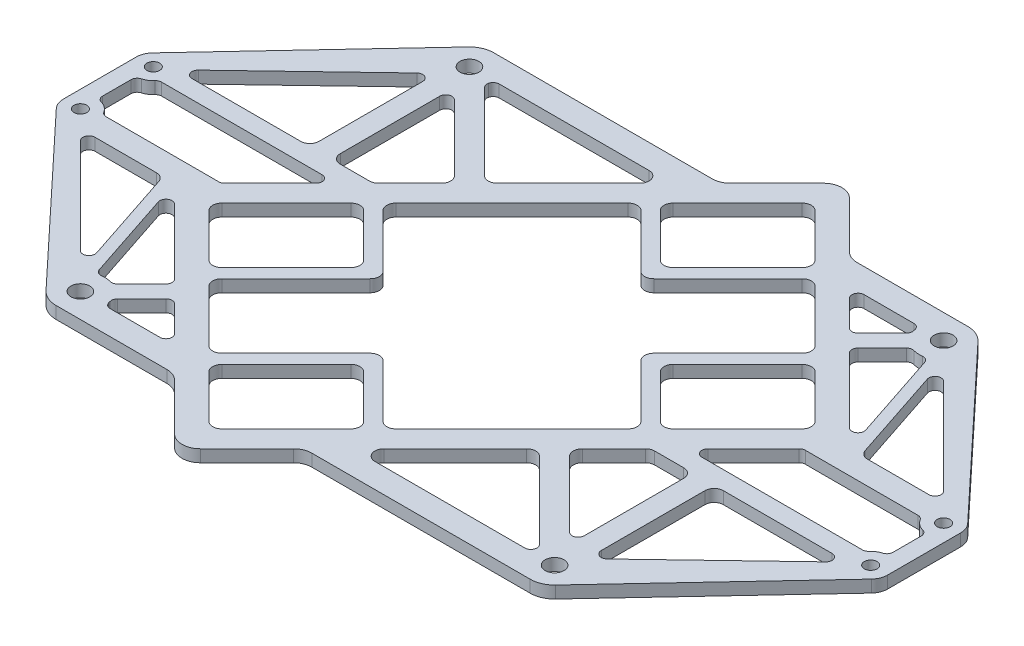
from build123d import *

# Parameters (mm, degrees)
SKETCH_1_R      = 2.8
SKETCH_1_R_2    = 1.05
SKETCH_1_R_3    = 4
SKETCH_1_R_4    = 1.55
EXTRUDE_1_DEPTH = 2
EXTRUDE_2_DEPTH = 2
FILLET_1_5_R    = 1.5
FILLET_1_R      = 1
FILLET_3_R      = 3


with BuildPart() as part:
    # 草图1 → 凸台-拉伸1 (new body)
    # profile 1 of 33: a face of its own
    with BuildSketch(Plane(origin=(0, 0, 0), x_dir=(1, 0, 0), z_dir=(0, 1, 0))):
        with BuildLine():
            ThreePointArc((-65, 3.2), (-66.979898987, 4.020101013), (-67.8, 6))
            Line((-67.8, 6), (-67.8, -6))
            ThreePointArc((-67.8, -6), (-66.979898987, -4.020101013), (-65, -3.2))
            Line((-65, -3.2), (-65, 3.2))
        make_face()
    # profile 2 of 33: a face of its own
    with BuildSketch(Plane(origin=(0, 0, 0), x_dir=(1, 0, 0), z_dir=(0, 1, 0))):
        with Locations((-65, 6)):
            Circle(SKETCH_1_R)
        with Locations(Location((-65, 6, 0), (0, 0, 270))):
            Circle(SKETCH_1_R_2, mode=Mode.SUBTRACT)
    # profile 3 of 33: a face of its own
    with BuildSketch(Plane(origin=(0, 0, 0), x_dir=(1, 0, 0), z_dir=(0, 1, 0))):
        with BuildLine():
            ThreePointArc((-40.75, 28.403126358), (-42.933491188, 31.273606806), (-41.919228153, 34.734612768))
            Line((-41.919228153, 34.734612768), (-67.043459707, 7.914228938))
            ThreePointArc((-67.043459707, 7.914228938), (-64.738019223, 8.787717), (-62.635681916, 7.5))
            Line((-62.635681916, 7.5), (-40.75, 28.403126358))
        make_face()
    # profile 4 of 33: a face of its own
    with BuildSketch(Plane(origin=(0, 0, 0), x_dir=(1, 0, 0), z_dir=(0, 1, 0))):
        with BuildLine():
            Line((-33.330212793, 4.5), (-30.330212793, 7.5))
            Line((-30.330212793, 7.5), (-37.25, 7.5))
            Line((-37.25, 7.5), (-40.75, 7.5))
            Line((-40.75, 7.5), (-62.635681916, 7.5))
            ThreePointArc((-62.635681916, 7.5), (-62.311125641, 6.780995956), (-62.2, 6))
            ThreePointArc((-62.2, 6), (-62.311125641, 5.219004044), (-62.635681916, 4.5))
            Line((-62.635681916, 4.5), (-33.330212793, 4.5))
        make_face()
    # profile 5 of 33: a face of its own
    with BuildSketch(Plane(origin=(0, 0, 0), x_dir=(1, 0, 0), z_dir=(0, 1, 0))):
        with Locations((-65, -6)):
            Circle(SKETCH_1_R)
        with Locations(Location((-65, -6, 0), (0, 0, 270))):
            Circle(SKETCH_1_R_2, mode=Mode.SUBTRACT)
    # profile 6 of 33: a face of its own
    with BuildSketch(Plane(origin=(0, 0, 0), x_dir=(1, 0, 0), z_dir=(0, 1, 0))):
        with BuildLine():
            Line((-46.669047558, -8.838834765), (-42.830212793, -5))
            Line((-42.830212793, -5), (-62.384660634, -5))
            ThreePointArc((-62.384660634, -5), (-62.246552141, -5.491546573), (-62.2, -6))
            ThreePointArc((-62.2, -6), (-62.413137309, -7.071513611), (-63.020101013, -7.979898987))
            Line((-63.020101013, -7.979898987), (-62.161165235, -8.838834765))
            Line((-62.161165235, -8.838834765), (-48.560935355, -8.838834765))
            Line((-48.560935355, -8.838834765), (-46.669047558, -8.838834765))
        make_face()
    # profile 7 of 33: a face of its own
    with BuildSketch(Plane(origin=(0, 0, 0), x_dir=(1, 0, 0), z_dir=(0, 1, 0))):
        with BuildLine():
            Line((-67.043459707, -7.914228938), (-41.919228153, -34.734612768))
            ThreePointArc((-41.919228153, -34.734612768), (-42.999467278, -31.934719911), (-41.828427125, -29.171572875))
            Line((-41.828427125, -29.171572875), (-62.161165235, -8.838834765))
            Line((-62.161165235, -8.838834765), (-63.020101013, -7.979898987))
            ThreePointArc((-63.020101013, -7.979898987), (-65.045696062, -8.799627095), (-67.043459707, -7.914228938))
        make_face()
    # profile 8 of 33: a face of its own
    with BuildSketch(Plane(origin=(0, 0, 0), x_dir=(1, 0, 0), z_dir=(0, 1, 0))):
        with BuildLine():
            Line((-48.560935355, -8.838834765), (-41.828427125, -29.171572875))
            ThreePointArc((-41.828427125, -29.171572875), (-41.099527033, -28.595299391), (-40.257332988, -28.202749184))
            Line((-40.257332988, -28.202749184), (-46.669047558, -8.838834765))
            Line((-46.669047558, -8.838834765), (-48.560935355, -8.838834765))
        make_face()
    # profile 9 of 33: a face of its own
    with BuildSketch(Plane(origin=(0, 0, 0), x_dir=(1, 0, 0), z_dir=(0, 1, 0))):
        Polygon((46.669047558, 8.838834765), (8.838834765, 46.669047558), (-46.669047558, -8.838834765), (-8.838834765, -46.669047558), align=None)
        Polygon((41.012193309, 8.838834765), (8.838834765, 41.012193309), (-41.012193309, -8.838834765), (-8.838834765, -41.012193309), align=None, mode=Mode.SUBTRACT)
    # profile 10 of 33: a face of its own
    with BuildSketch(Plane(origin=(0, 0, 0), x_dir=(1, 0, 0), z_dir=(0, 1, 0))):
        with Locations((-39, 32)):
            Circle(SKETCH_1_R_3)
        with Locations(Location((-39, 32, 0), (0, 0, 270))):
            Circle(SKETCH_1_R_4, mode=Mode.SUBTRACT)
    # profile 11 of 33: a face of its own
    with BuildSketch(Plane(origin=(0, 0, 0), x_dir=(1, 0, 0), z_dir=(0, 1, 0))):
        with BuildLine():
            ThreePointArc((-37.694063123, 28.219189389), (-39.240325231, 28.007226054), (-40.75, 28.403126358))
            Line((-40.75, 28.403126358), (-40.75, 7.5))
            Line((-40.75, 7.5), (-37.25, 7.5))
            Line((-37.25, 7.5), (-37.25, 27.775126266))
            Line((-37.25, 27.775126266), (-37.694063123, 28.219189389))
        make_face()
    # profile 12 of 33: a face of its own
    with BuildSketch(Plane(origin=(0, 0, 0), x_dir=(1, 0, 0), z_dir=(0, 1, 0))):
        with BuildLine():
            Line((-37.694063123, 28.219189389), (-37.25, 27.775126266))
            Line((-37.25, 27.775126266), (-37.25, 28.403126358))
            ThreePointArc((-37.25, 28.403126358), (-37.469266271, 28.30448187), (-37.694063123, 28.219189389))
        make_face()
    # profile 13 of 33: a face of its own
    with BuildSketch(Plane(origin=(0, 0, 0), x_dir=(1, 0, 0), z_dir=(0, 1, 0))):
        with BuildLine():
            Line((-23.652543264, 14.17766953), (-21.17766953, 16.652543264))
            Line((-21.17766953, 16.652543264), (-35.219189389, 30.694063123))
            ThreePointArc((-35.219189389, 30.694063123), (-36.006746867, 29.346618067), (-37.25, 28.403126358))
            Line((-37.25, 28.403126358), (-37.25, 27.775126266))
            Line((-37.25, 27.775126266), (-23.652543264, 14.17766953))
        make_face()
    # profile 14 of 33: a face of its own
    with BuildSketch(Plane(origin=(0, 0, 0), x_dir=(1, 0, 0), z_dir=(0, 1, 0))):
        with BuildLine():
            Line((-5.830212793, 32), (-1.830212793, 36))
            Line((-1.830212793, 36), (-39, 36))
            ThreePointArc((-39, 36), (-36.171572875, 34.828427125), (-35, 32))
            Line((-35, 32), (-5.830212793, 32))
        make_face()
    # profile 15 of 33: a face of its own
    with BuildSketch(Plane(origin=(0, 0, 0), x_dir=(1, 0, 0), z_dir=(0, 1, 0))):
        with Locations((-39, -32)):
            Circle(SKETCH_1_R_3)
        with Locations(Location((-39, -32, 0), (0, 0, 270))):
            Circle(SKETCH_1_R_4, mode=Mode.SUBTRACT)
    # profile 16 of 33: a face of its own
    with BuildSketch(Plane(origin=(0, 0, 0), x_dir=(1, 0, 0), z_dir=(0, 1, 0))):
        with BuildLine():
            Line((-35.317317708, -30.438638051), (-30.19328099, -25.314601333))
            Line((-30.19328099, -25.314601333), (-32.314601333, -23.19328099))
            Line((-32.314601333, -23.19328099), (-37.438638051, -28.317317708))
            ThreePointArc((-37.438638051, -28.317317708), (-36.171572875, -29.171572875), (-35.317317708, -30.438638051))
        make_face()
    # profile 17 of 33: a face of its own
    with BuildSketch(Plane(origin=(0, 0, 0), x_dir=(1, 0, 0), z_dir=(0, 1, 0))):
        with BuildLine():
            Line((-39, -36), (-19.507882323, -36))
            Line((-19.507882323, -36), (-23.507882323, -32))
            Line((-23.507882323, -32), (-35, -32))
            ThreePointArc((-35, -32), (-36.171572875, -34.828427125), (-39, -36))
        make_face()
    # profile 18 of 33: a face of its own
    with BuildSketch(Plane(origin=(0, 0, 0), x_dir=(1, 0, 0), z_dir=(0, 1, 0))):
        with BuildLine():
            Line((35, -32), (5.830212793, -32))
            Line((5.830212793, -32), (1.830212793, -36))
            Line((1.830212793, -36), (39, -36))
            ThreePointArc((39, -36), (36.171572875, -34.828427125), (35, -32))
        make_face()
    # profile 19 of 33: a face of its own
    with BuildSketch(Plane(origin=(0, 0, 0), x_dir=(1, 0, 0), z_dir=(0, 1, 0))):
        with BuildLine():
            Line((37.25, -27.775126266), (23.652543264, -14.17766953))
            Line((23.652543264, -14.17766953), (21.17766953, -16.652543264))
            Line((21.17766953, -16.652543264), (35.219189389, -30.694063123))
            ThreePointArc((35.219189389, -30.694063123), (36.006746867, -29.346618067), (37.25, -28.403126358))
            Line((37.25, -28.403126358), (37.25, -27.775126266))
        make_face()
    # profile 20 of 33: a face of its own
    with BuildSketch(Plane(origin=(0, 0, 0), x_dir=(1, 0, 0), z_dir=(0, 1, 0))):
        with BuildLine():
            Line((40.75, -7.5), (37.25, -7.5))
            Line((37.25, -7.5), (37.25, -27.775126266))
            Line((37.25, -27.775126266), (37.694063123, -28.219189389))
            ThreePointArc((37.694063123, -28.219189389), (39.240325231, -28.007226054), (40.75, -28.403126358))
            Line((40.75, -28.403126358), (40.75, -7.5))
        make_face()
    # profile 21 of 33: a face of its own
    with BuildSketch(Plane(origin=(0, 0, 0), x_dir=(1, 0, 0), z_dir=(0, 1, 0))):
        with Locations((39, -32)):
            Circle(SKETCH_1_R_3)
        with Locations(Location((39, -32, 0), (0, 0, 270))):
            Circle(SKETCH_1_R_4, mode=Mode.SUBTRACT)
    # profile 22 of 33: a face of its own
    with BuildSketch(Plane(origin=(0, 0, 0), x_dir=(1, 0, 0), z_dir=(0, 1, 0))):
        with BuildLine():
            Line((37.694063123, -28.219189389), (37.25, -27.775126266))
            Line((37.25, -27.775126266), (37.25, -28.403126358))
            ThreePointArc((37.25, -28.403126358), (37.469266271, -28.30448187), (37.694063123, -28.219189389))
        make_face()
    # profile 23 of 33: a face of its own
    with BuildSketch(Plane(origin=(0, 0, 0), x_dir=(1, 0, 0), z_dir=(0, 1, 0))):
        with BuildLine():
            ThreePointArc((67.043459707, -7.914228938), (64.738019223, -8.787717), (62.635681916, -7.5))
            Line((62.635681916, -7.5), (40.75, -28.403126358))
            ThreePointArc((40.75, -28.403126358), (42.391164992, -29.878679656), (43, -32))
            ThreePointArc((43, -32), (42.720007568, -33.470218927), (41.919228153, -34.734612768))
            Line((41.919228153, -34.734612768), (67.043459707, -7.914228938))
        make_face()
    # profile 24 of 33: a face of its own
    with BuildSketch(Plane(origin=(0, 0, 0), x_dir=(1, 0, 0), z_dir=(0, 1, 0))):
        with Locations((65, -6)):
            Circle(SKETCH_1_R)
        with Locations(Location((65, -6, 0), (0, 0, 270))):
            Circle(SKETCH_1_R_2, mode=Mode.SUBTRACT)
    # profile 25 of 33: a face of its own
    with BuildSketch(Plane(origin=(0, 0, 0), x_dir=(1, 0, 0), z_dir=(0, 1, 0))):
        with BuildLine():
            Line((62.635681916, -4.5), (33.330212793, -4.5))
            Line((33.330212793, -4.5), (30.330212793, -7.5))
            Line((30.330212793, -7.5), (37.25, -7.5))
            Line((37.25, -7.5), (40.75, -7.5))
            Line((40.75, -7.5), (62.635681916, -7.5))
            ThreePointArc((62.635681916, -7.5), (62.2, -6), (62.635681916, -4.5))
        make_face()
    # profile 26 of 33: a face of its own
    with BuildSketch(Plane(origin=(0, 0, 0), x_dir=(1, 0, 0), z_dir=(0, 1, 0))):
        with BuildLine():
            ThreePointArc((67.8, 6), (66.979898987, 4.020101013), (65, 3.2))
            Line((65, 3.2), (65, -3.2))
            ThreePointArc((65, -3.2), (66.979898987, -4.020101013), (67.8, -6))
            Line((67.8, -6), (67.8, 6))
        make_face()
    # profile 27 of 33: a face of its own
    with BuildSketch(Plane(origin=(0, 0, 0), x_dir=(1, 0, 0), z_dir=(0, 1, 0))):
        with BuildLine():
            Line((48.560935355, 8.838834765), (46.669047558, 8.838834765))
            Line((46.669047558, 8.838834765), (42.830212793, 5))
            Line((42.830212793, 5), (62.384660634, 5))
            ThreePointArc((62.384660634, 5), (62.261569177, 6.583949163), (63.020101013, 7.979898987))
            Line((63.020101013, 7.979898987), (62.161165235, 8.838834765))
            Line((62.161165235, 8.838834765), (48.560935355, 8.838834765))
        make_face()
    # profile 28 of 33: a face of its own
    with BuildSketch(Plane(origin=(0, 0, 0), x_dir=(1, 0, 0), z_dir=(0, 1, 0))):
        with BuildLine():
            Line((41.828427125, 29.171572875), (62.161165235, 8.838834765))
            Line((62.161165235, 8.838834765), (63.020101013, 7.979898987))
            ThreePointArc((63.020101013, 7.979898987), (65.045696062, 8.799627095), (67.043459707, 7.914228938))
            Line((67.043459707, 7.914228938), (41.919228153, 34.734612768))
            ThreePointArc((41.919228153, 34.734612768), (42.720007568, 33.470218927), (43, 32))
            ThreePointArc((43, 32), (42.69551813, 30.469266271), (41.828427125, 29.171572875))
        make_face()
    # profile 29 of 33: a face of its own
    with BuildSketch(Plane(origin=(0, 0, 0), x_dir=(1, 0, 0), z_dir=(0, 1, 0))):
        with Locations((65, 6)):
            Circle(SKETCH_1_R)
        with Locations(Location((65, 6, 0), (0, 0, 270))):
            Circle(SKETCH_1_R_2, mode=Mode.SUBTRACT)
    # profile 30 of 33: a face of its own
    with BuildSketch(Plane(origin=(0, 0, 0), x_dir=(1, 0, 0), z_dir=(0, 1, 0))):
        with BuildLine():
            Line((40.257332988, 28.202749184), (46.669047558, 8.838834765))
            Line((46.669047558, 8.838834765), (48.560935355, 8.838834765))
            Line((48.560935355, 8.838834765), (41.828427125, 29.171572875))
            ThreePointArc((41.828427125, 29.171572875), (41.099527033, 28.595299391), (40.257332988, 28.202749184))
        make_face()
    # profile 31 of 33: a face of its own
    with BuildSketch(Plane(origin=(0, 0, 0), x_dir=(1, 0, 0), z_dir=(0, 1, 0))):
        with BuildLine():
            Line((19.507882323, 36), (23.507882323, 32))
            Line((23.507882323, 32), (35, 32))
            ThreePointArc((35, 32), (36.171572875, 34.828427125), (39, 36))
            Line((39, 36), (19.507882323, 36))
        make_face()
    # profile 32 of 33: a face of its own
    with BuildSketch(Plane(origin=(0, 0, 0), x_dir=(1, 0, 0), z_dir=(0, 1, 0))):
        with Locations((39, 32)):
            Circle(SKETCH_1_R_3)
        with Locations(Location((39, 32, 0), (0, 0, 270))):
            Circle(SKETCH_1_R_4, mode=Mode.SUBTRACT)
    # profile 33 of 33: a face of its own
    with BuildSketch(Plane(origin=(0, 0, 0), x_dir=(1, 0, 0), z_dir=(0, 1, 0))):
        with BuildLine():
            Line((30.19328099, 25.314601333), (32.314601333, 23.19328099))
            Line((32.314601333, 23.19328099), (37.438638051, 28.317317708))
            ThreePointArc((37.438638051, 28.317317708), (36.171572875, 29.171572875), (35.317317708, 30.438638051))
            Line((35.317317708, 30.438638051), (30.19328099, 25.314601333))
        make_face()
    extrude(amount=EXTRUDE_1_DEPTH)

    # 草图2 → 凸台-拉伸2 (add)
    with BuildSketch(Plane(origin=(0, 2, 0), x_dir=(1, 0, 0), z_dir=(0, 1, 0))):
        Polygon((-3.889087297, 28.284271247), (5.303300859, 19.091883092), (18.03122292, 31.819805153), (19.622213178, 30.228814896), (5.303300859, 15.909902577), (-5.480077554, 26.69328099), align=None)
        Polygon((-31.819805153, -18.03122292), (-30.228814896, -19.622213178), (-15.909902577, -5.303300859), (-26.69328099, 5.480077554), (-28.284271247, 3.889087297), (-19.091883092, -5.303300859), align=None)
        Polygon((31.819805153, 18.03122292), (30.228814896, 19.622213178), (15.909902577, 5.303300859), (26.69328099, -5.480077554), (28.284271247, -3.889087297), (19.091883092, 5.303300859), align=None)
        Polygon((5.480077554, -26.69328099), (-5.303300859, -15.909902577), (-19.622213178, -30.228814896), (-18.03122292, -31.819805153), (-5.303300859, -19.091883092), (3.889087297, -28.284271247), align=None)
    extrude(amount=-EXTRUDE_2_DEPTH)

    # 1.5
    fillet_1_5_edges = [part.edges().sort_by_distance(p)[0] for p in [
        (8.838834765, 1, -41.012193309),
        (-41.012193309, 1, 8.838834765),
        (-8.838834765, 1, 41.012193309),
        (41.012193309, 1, -8.838834765),
        (-40.75, 1, -7.5),
        (21.17766953, 1, 16.652543264),
        (5.830212793, 1, 32),
        (-21.17766953, 1, -16.652543264),
        (-5.830212793, 1, -32),
        (-48.560935355, 1, 8.838834765),
        (-37.25, 1, -7.5),
        (-30.330212793, 1, -7.5),
        (-23.652543264, 1, -14.17766953),
        (48.560935355, 1, -8.838834765),
        (37.25, 1, 7.5),
        (30.330212793, 1, 7.5),
        (23.652543264, 1, 14.17766953),
        (40.75, 1, 7.5),
        (-5.480077554, 1, -26.69328099),
        (-3.889087297, 1, -28.284271247),
        (5.303300859, 1, -19.091883092),
        (18.03122292, 1, -31.819805153),
        (19.622213178, 1, -30.228814896),
        (5.303300859, 1, -15.909902577),
        (-31.819805153, 1, 18.03122292),
        (-19.091883092, 1, 5.303300859),
        (-28.284271247, 1, -3.889087297),
        (-26.69328099, 1, -5.480077554),
        (-15.909902577, 1, 5.303300859),
        (-30.228814896, 1, 19.622213178),
        (31.819805153, 1, -18.03122292),
        (19.091883092, 1, -5.303300859),
        (28.284271247, 1, 3.889087297),
        (26.69328099, 1, 5.480077554),
        (15.909902577, 1, -5.303300859),
        (30.228814896, 1, -19.622213178),
        (5.480077554, 1, 26.69328099),
        (3.889087297, 1, 28.284271247),
        (-5.303300859, 1, 19.091883092),
        (-18.03122292, 1, 31.819805153),
        (-19.622213178, 1, 30.228814896),
        (-5.303300859, 1, 15.909902577),
    ]]
    fillet(fillet_1_5_edges, radius=FILLET_1_5_R)

    # 1
    fillet_1_edges = [part.edges().sort_by_distance(p)[0] for p in [
        (-33.330212793, 1, -4.5),
        (-62.635681916, 1, -4.5),
        (-65, 1, -3.2),
        (-65, 1, 3.2),
        (-62.384660634, 1, 5),
        (-42.830212793, 1, 5),
        (-62.635681916, 1, -7.5),
        (-40.75, 1, -28.403126358),
        (35.219189389, 1, 30.694063123),
        (35, 1, 32),
        (-35, 1, -32),
        (-35.219189389, 1, -30.694063123),
        (-62.161165235, 1, 8.838834765),
        (-41.828427125, 1, 29.171572875),
        (-32.314601333, 1, 23.19328099),
        (-46.669047558, 1, 8.838834765),
        (-40.257332988, 1, 28.202749184),
        (-37.438638051, 1, 28.317317708),
        (-23.507882323, 1, 32),
        (-30.19328099, 1, 25.314601333),
        (-35.317317708, 1, 30.438638051),
        (-35, 1, 32),
        (-37.25, 1, -27.775126266),
        (37.438638051, 1, -28.317317708),
        (32.314601333, 1, -23.19328099),
        (46.669047558, 1, -8.838834765),
        (40.257332988, 1, -28.202749184),
        (23.507882323, 1, -32),
        (30.19328099, 1, -25.314601333),
        (35.317317708, 1, -30.438638051),
        (35, 1, -32),
        (62.161165235, 1, -8.838834765),
        (41.828427125, 1, -29.171572875),
        (37.25, 1, 27.775126266),
        (65, 1, -3.2),
        (62.384660634, 1, -5),
        (42.830212793, 1, -5),
        (33.330212793, 1, 4.5),
        (62.635681916, 1, 4.5),
        (65, 1, 3.2),
        (62.635681916, 1, 7.5),
        (40.75, 1, 28.403126358),
    ]]
    fillet(fillet_1_edges, radius=FILLET_1_R)

    # 3
    fillet_3_edges = [part.edges().sort_by_distance(p)[0] for p in [
        (1.830212793, 1, 36),
        (-8.838834765, 1, 46.669047558),
        (-19.507882323, 1, 36),
        (-1.830212793, 1, -36),
        (8.838834765, 1, -46.669047558),
        (19.507882323, 1, -36),
    ]]
    fillet(fillet_3_edges, radius=FILLET_3_R)


solid = part.part
